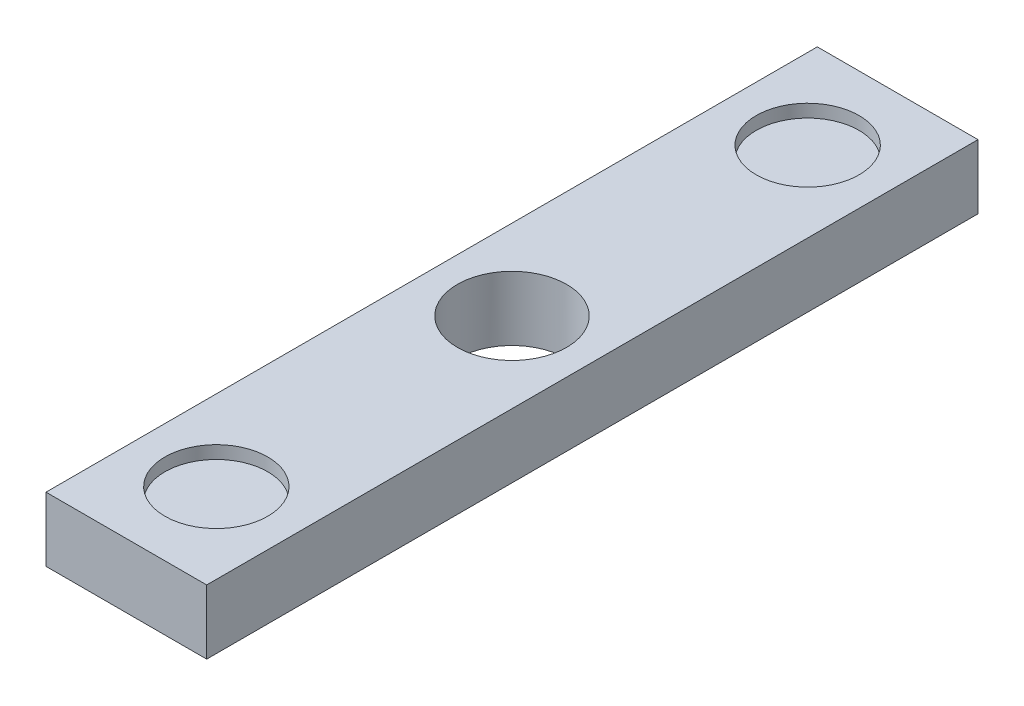
from build123d import *

# Parameters (mm, degrees)
SKETCH_1_W          = 25
SKETCH_1_H          = 120
EXTRUDE_1_DEPTH     = 10
SKETCH_2_R          = 8
CUT_EXTRUDE_1_DEPTH = 2
CUT_EXTRUDE_2_REACH = 64.099
SKETCH_3_R          = 8.5


with BuildPart() as part:
    # 草图1 → 凸台-拉伸1 (new body)
    with BuildSketch(Plane(origin=(0, 0, 0), x_dir=(1, 0, 0), z_dir=(0, 1, 0))):
        Rectangle(SKETCH_1_W, SKETCH_1_H)
    extrude(amount=EXTRUDE_1_DEPTH)

    # 草图2 → 切除-拉伸1 (cut)
    with BuildSketch(Plane(origin=(0, 10, 0), x_dir=(1, 0, 0), z_dir=(0, 1, 0))):
        with Locations(Location((0, 46, 0), (0, 0, 270))):
            Circle(SKETCH_2_R)
        with Locations(Location((0, -46, 0), (0, 0, 270))):
            Circle(SKETCH_2_R)
    extrude(amount=-CUT_EXTRUDE_1_DEPTH, mode=Mode.SUBTRACT)

    # 草图3 → 切除-拉伸2 (cut, up to next)
    with BuildSketch(Plane(origin=(0, 10, 0), x_dir=(1, 0, 0), z_dir=(0, 1, 0)), mode=Mode.PRIVATE) as cut_extrude_2_sk1:
        with Locations(Location((0, 0, 0), (0, 0, 270))):
            Circle(SKETCH_3_R)
    cut_extrude_2_tool1 = extrude(cut_extrude_2_sk1.sketch, amount=-CUT_EXTRUDE_2_REACH, mode=Mode.PRIVATE) & part.part
    add(cut_extrude_2_tool1.solids().sort_by_distance((0, 10, 0))[0], mode=Mode.SUBTRACT)


solid = part.part
